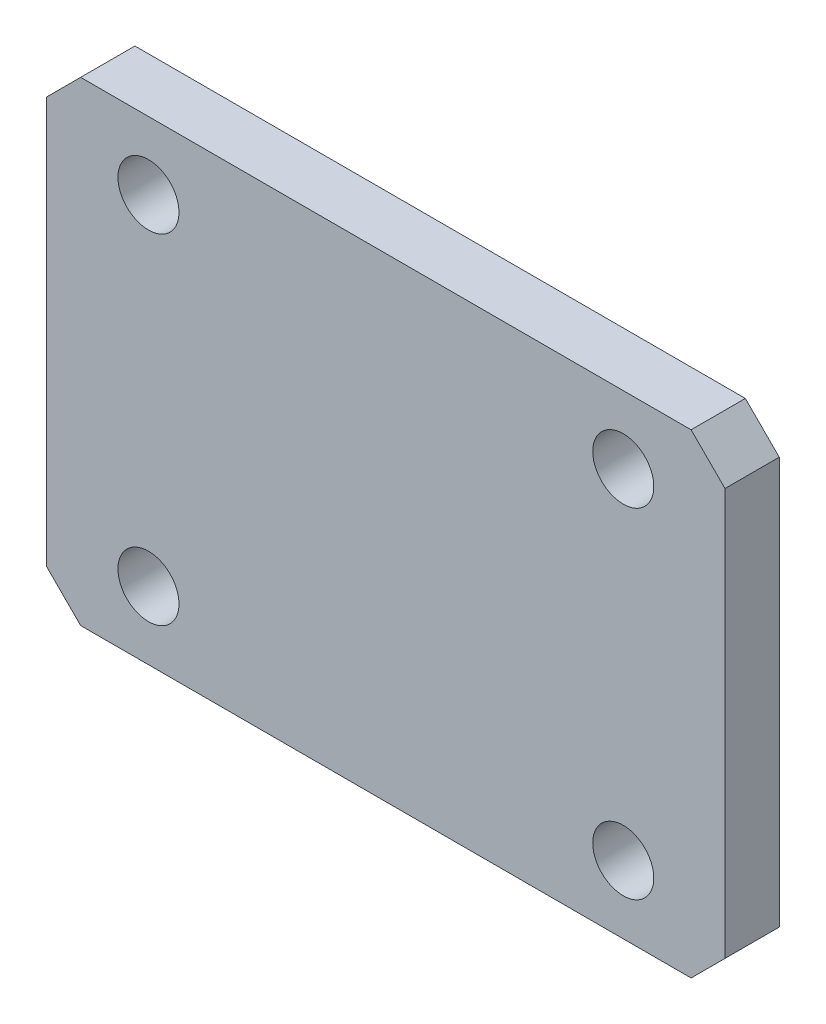
from build123d import *

# Parameters (mm, degrees)
SKETCH1_W           = 100
SKETCH1_H           = 70
BOSS_EXTRUDE1_DEPTH = 8
SKETCH2_R           = 4.5
CUT_EXTRUDE1_DEPTH  = 8
CHAMFER1_SIZE       = 5


with BuildPart() as part:
    # Sketch1 → Boss-Extrude1 (new body)
    with BuildSketch(Plane.XY.offset(-15)):
        with Locations((0, -175)):
            Rectangle(SKETCH1_W, SKETCH1_H)
    extrude(amount=-BOSS_EXTRUDE1_DEPTH)

    # Sketch2 → Cut-Extrude1 (cut)
    with BuildSketch(Plane(origin=(0, 0, -23), x_dir=(-1, 0, 0), z_dir=(0, 0, -1))):
        with Locations((-35, -150)):
            Circle(SKETCH2_R)
        with Locations((35, -150)):
            Circle(SKETCH2_R)
        with Locations((35, -200)):
            Circle(SKETCH2_R)
        with Locations((-35, -200)):
            Circle(SKETCH2_R)
    extrude(amount=-CUT_EXTRUDE1_DEPTH, mode=Mode.SUBTRACT)

    # Chamfer1
    chamfer1_edges = [part.edges().sort_by_distance(p)[0] for p in [
        (50, -210, -19),
        (-50, -210, -19),
        (-50, -140, -19),
        (50, -140, -19),
    ]]
    chamfer(chamfer1_edges, length=CHAMFER1_SIZE)


solid = part.part
